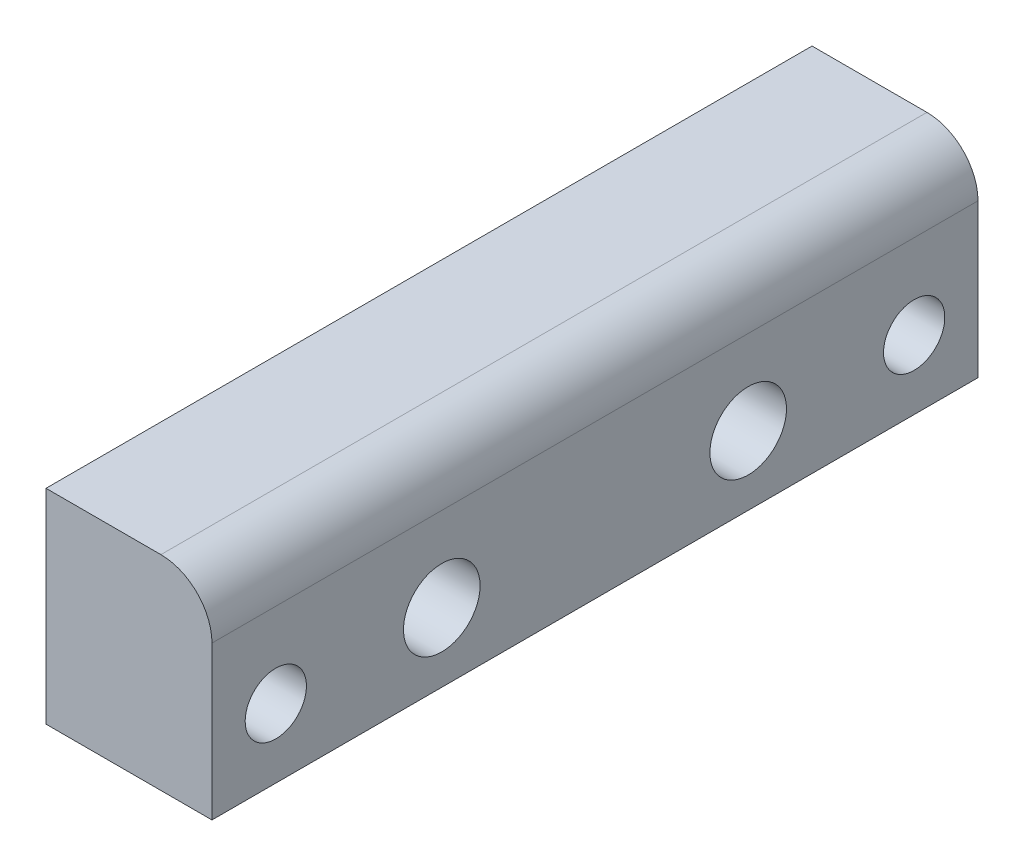
from build123d import *

# Parameters (mm, degrees)
SKETCH_1_W                   = 30
SKETCH_1_H                   = 8
EXTRUDE_1_DEPTH              = 6.5
HOLE_WIZARD_3_0_3_1_D        = 3
HOLE_WIZARD_3_0_3_1_DEPTH    = 3
HOLE_WIZARD_M2_1_D           = 2.4
HOLE_WIZARD_M2_1_CBORE_D     = 4.3
HOLE_WIZARD_M2_1_CBORE_DEPTH = 2
CHAMFER_1_SIZE               = 0.1
CHAMFER_1_SIZE2              = 0.096568877
FILLET_1_R                   = 2


with BuildPart() as part:
    # 草图1 → 凸台-拉伸1 (new body)
    with BuildSketch(Plane(origin=(3.25, 0, 0), x_dir=(0, 0, -1), z_dir=(1, 0, 0))):
        with Locations((-15, 0)):
            Rectangle(SKETCH_1_W, SKETCH_1_H)
    extrude(amount=-EXTRUDE_1_DEPTH)

    # Ø3.0 (3) 直径孔1
    with Locations(Plane(origin=(3.25, 0, 0), x_dir=(0, 0, -1), z_dir=(1, 0, 0))):
        with Locations((-9, -1.3), (-21, -1.3)):
            Hole(HOLE_WIZARD_3_0_3_1_D / 2, depth=HOLE_WIZARD_3_0_3_1_DEPTH)

    # M2 六角头机械螺钉的柱形沉头孔1 (through all)
    with Locations(Plane.ZY.offset(3.25)):
        with Locations((27.5, -1.3), (2.5, -1.3)):
            CounterBoreHole(HOLE_WIZARD_M2_1_D / 2, HOLE_WIZARD_M2_1_CBORE_D / 2, HOLE_WIZARD_M2_1_CBORE_DEPTH)

    # 倒角1
    chamfer_1_edges = [part.edges().sort_by_distance(p)[0] for p in [
        (-3.25, -1.3, 0.35),
        (-3.25, -1.3, 25.35),
    ]]
    chamfer_1_side = [part.faces().sort_by_distance(p)[0] for p in [
        (-3.25, 0.178981568, 15),
    ]]
    chamfer(chamfer_1_edges, length=CHAMFER_1_SIZE, length2=CHAMFER_1_SIZE2, reference=chamfer_1_side[0])

    # 圆角1
    fillet_1_edges = [part.edges().sort_by_distance(p)[0] for p in [
        (3.25, 4, 15),
    ]]
    fillet(fillet_1_edges, radius=FILLET_1_R)


solid = part.part
